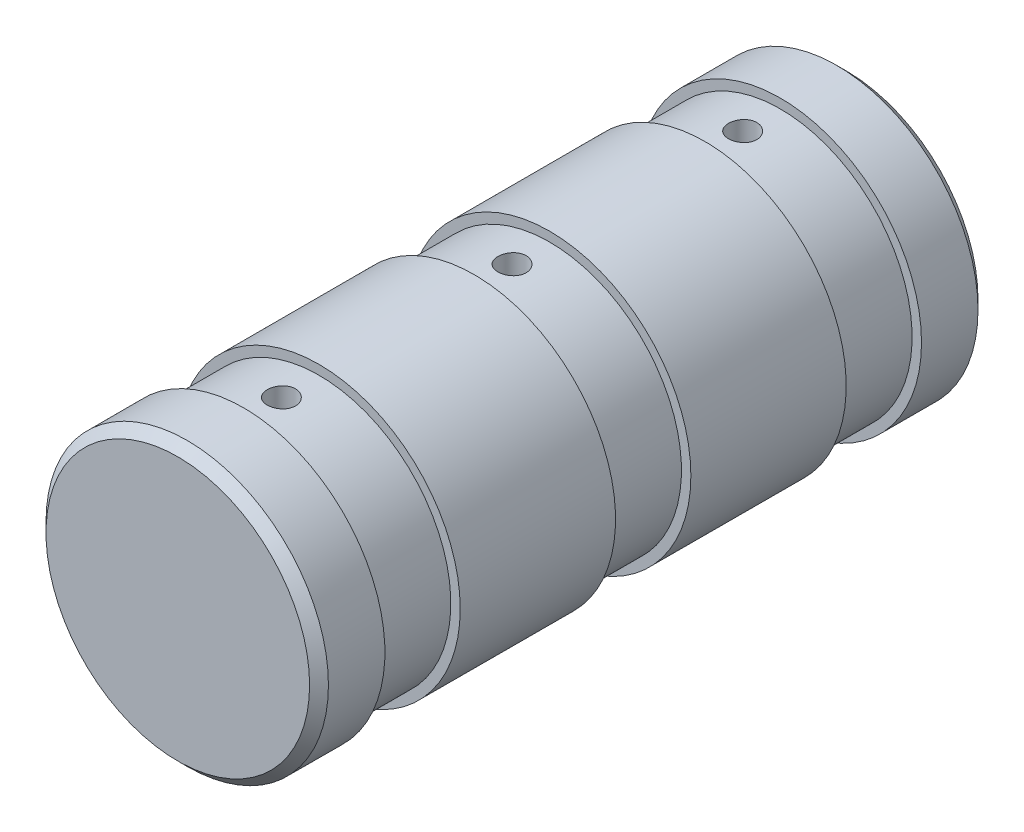
from build123d import *

# Parameters (mm, degrees)
SKETCH1_R                  = 15
BOSS_EXTRUDE1_DEPTH        = 71
CHAMFER1_SIZE              = 1
SKETCH6_R                  = 1.5
CUT_EXTRUDE1_DEPTH         = 17
SIZE_MM_DOWEL_HOLE_6_D     = 3
SIZE_MM_DOWEL_HOLE_6_DEPTH = 17
SIZE_MM_DOWEL_HOLE_6_TIP   = 0.901290929
SKETCH17_W                 = 2
SKETCH17_H                 = 8
SIZE_MM_DOWEL_HOLE_7_D     = 3
SIZE_MM_DOWEL_HOLE_7_DEPTH = 62
SIZE_MM_DOWEL_HOLE_7_TIP   = 0.901290929
M4_TAPPED_HOLE1_D          = 3.3
M4_TAPPED_HOLE1_DEPTH      = 5.008579979
M4_TAPPED_HOLE1_TIP        = 0.991420021


with BuildPart() as part:
    # Sketch1 → Boss-Extrude1 (new body)
    with BuildSketch(Plane.XY):
        Circle(SKETCH1_R)
    extrude(amount=BOSS_EXTRUDE1_DEPTH)

    # Chamfer1
    chamfer1_edges = [part.edges().sort_by_distance(p)[0] for p in [
        (-15, 0, 0),
        (-15, 0, 71),
    ]]
    chamfer(chamfer1_edges, length=CHAMFER1_SIZE)

    # Sketch6 → Cut-Extrude1 (cut)
    with BuildSketch(Plane(origin=(0, 15, 0), x_dir=(1, 0, 0), z_dir=(0, 1, 0))):
        with Locations(Location((0, -11, 0), (0, 0, 270))):
            Circle(SKETCH6_R)
        with Locations(Location((0, -35.5, 0), (0, 0, 270))):
            Circle(SKETCH6_R)
        with Locations(Location((0, -60, 0), (0, 0, 270))):
            Circle(SKETCH6_R)
    extrude(amount=-CUT_EXTRUDE1_DEPTH, mode=Mode.SUBTRACT)

    # Size mm dowel hole 6
    with Locations(Plane(origin=(0, 15, 0), x_dir=(1, 0, 0), z_dir=(0, 1, 0))):
        with Locations((0, -11), (0, -35.5), (0, -60)):
            Hole(SIZE_MM_DOWEL_HOLE_6_D / 2, depth=SIZE_MM_DOWEL_HOLE_6_DEPTH)
            with Locations((0, 0, -(SIZE_MM_DOWEL_HOLE_6_DEPTH + SIZE_MM_DOWEL_HOLE_6_TIP / 2))):  # 118° drill point
                Cone(0, SIZE_MM_DOWEL_HOLE_6_D / 2, SIZE_MM_DOWEL_HOLE_6_TIP, mode=Mode.SUBTRACT)

    # Sketch17 → Cut-Revolve1 (revolve, cut)
    with BuildSketch(Plane(origin=(0, 0, 0), x_dir=(1, 0, 0), z_dir=(0, 1, 0)), mode=Mode.PRIVATE) as cut_revolve1_sk:
        with Locations((15, -11)):
            Rectangle(SKETCH17_W, SKETCH17_H)
        with Locations((15, -35.5)):
            Rectangle(SKETCH17_W, SKETCH17_H)
        with Locations((15, -60)):
            Rectangle(SKETCH17_W, SKETCH17_H)
    revolve(cut_revolve1_sk.sketch.rotate(Axis((0, 0, 0), (0, 0, 1)), 180), axis=Axis((0, 0, 0), (0, 0, 1)), mode=Mode.SUBTRACT)

    # Size mm dowel hole 7
    with Locations(Plane(origin=(0, 0, 0), x_dir=(-1, 0, 0), z_dir=(0, 0, -1))):
        with Locations((0, 0)):
            Hole(SIZE_MM_DOWEL_HOLE_7_D / 2, depth=SIZE_MM_DOWEL_HOLE_7_DEPTH)
            with Locations((0, 0, -(SIZE_MM_DOWEL_HOLE_7_DEPTH + SIZE_MM_DOWEL_HOLE_7_TIP / 2))):  # 118° drill point
                Cone(0, SIZE_MM_DOWEL_HOLE_7_D / 2, SIZE_MM_DOWEL_HOLE_7_TIP, mode=Mode.SUBTRACT)

    # M4 Tapped Hole1
    with Locations(Plane(origin=(0, 0, 0), x_dir=(-1, 0, 0), z_dir=(0, 0, -1))):
        with Locations((0, 0)):
            Hole(M4_TAPPED_HOLE1_D / 2, depth=M4_TAPPED_HOLE1_DEPTH)
            with Locations((0, 0, -(M4_TAPPED_HOLE1_DEPTH + M4_TAPPED_HOLE1_TIP / 2))):  # 118° drill point
                Cone(0, M4_TAPPED_HOLE1_D / 2, M4_TAPPED_HOLE1_TIP, mode=Mode.SUBTRACT)


solid = part.part
